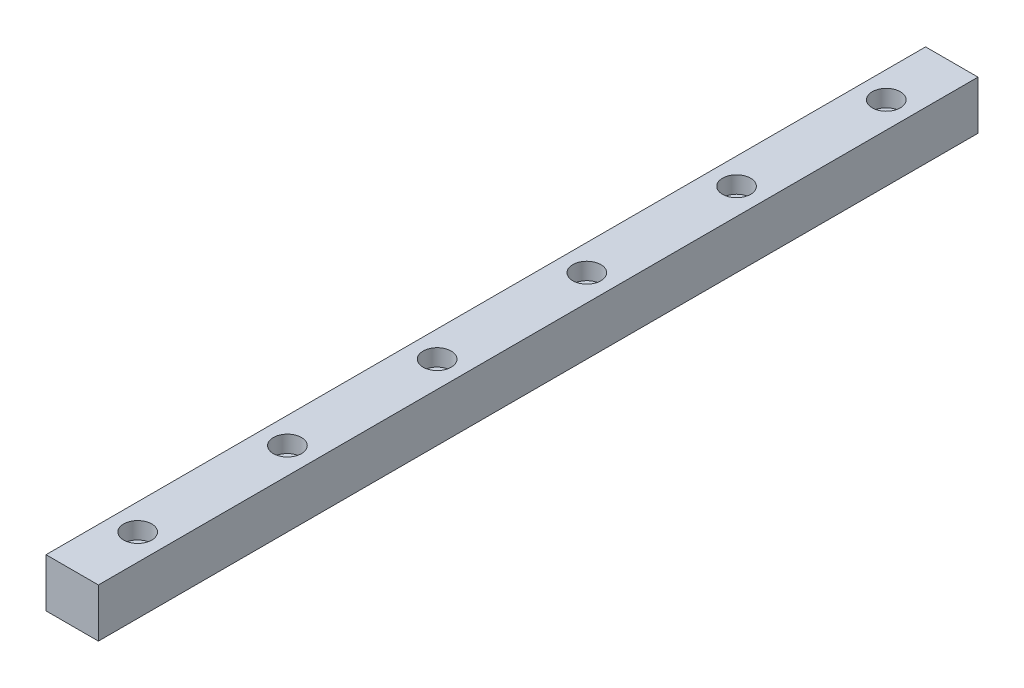
SolidWorks part; units mm, degrees
ref_plane "Front Plane" through (0, 0, 0) normal (0, 0, 1) x (1, 0, 0)
ref_plane "Top Plane" through (0, 0, 0) normal (0, 1, 0) x (1, 0, 0)
ref_plane "Right Plane" through (0, 0, 0) normal (1, 0, 0) x (0, 0, -1)
sketch "Sketch1" plane through (0, 0, 0) normal (0, 0, 1) x (1, 0, 0)
  line L1 (-14, 13) -> (14, 13)
  line L2 (-14, 13) -> (-14, -13)
  line L3 (-14, -13) -> (14, -13)
  line L4 (14, 13) -> (14, -13)
  line L5 (-14, 13) -> (14, -13) construction
  line L6 (-14, -13) -> (14, 13) construction
  point P0 (0, 0)
  dimension "D1" = 28
  dimension "D2" = 26
extrude "Boss-Extrude1" add sketch "Sketch1" against normal blind 470
hole_wizard "Hole size per socket head cap screw type1" positions "Sketch3" profile "Sketch2" counterbore size "M8" standard "GB" end condition through all
sketch "Sketch3" plane through (0, 13, 0) normal (0, 1, 0) x (-1, 0, 0)
  line L0 (-14, 0) -> (14, 0) construction
  point P1 (0, -35)
  dimension "D1" = 35
sketch "Sketch2" plane through (0, 13, -35) normal (1, 0, 0) x (0, 0, 1)
  line L0 (0, 0) -> (0, 26)
  line L1 (0, 26) -> (4.5, 26)
  line L3 (4.5, 26) -> (4.5, 9)
  line L4 (4.5, 9) -> (7.5, 9)
  line L5 (7.5, 9) -> (7.5, 0)
  line L7 (7.5, 0) -> (0, 0)
  line L11 (0, -6.35) -> (0, 107.95) construction
  dimension "通孔孔直径" = 9
  dimension "通孔孔深度" = 26
  dimension "柱形沉头孔直径" = 15
  dimension "柱形沉头孔深度" = 9
pattern_linear "LPattern1" count 6 spacing 80 along (0, 0, -1) of "Hole size per socket head cap screw type1"
